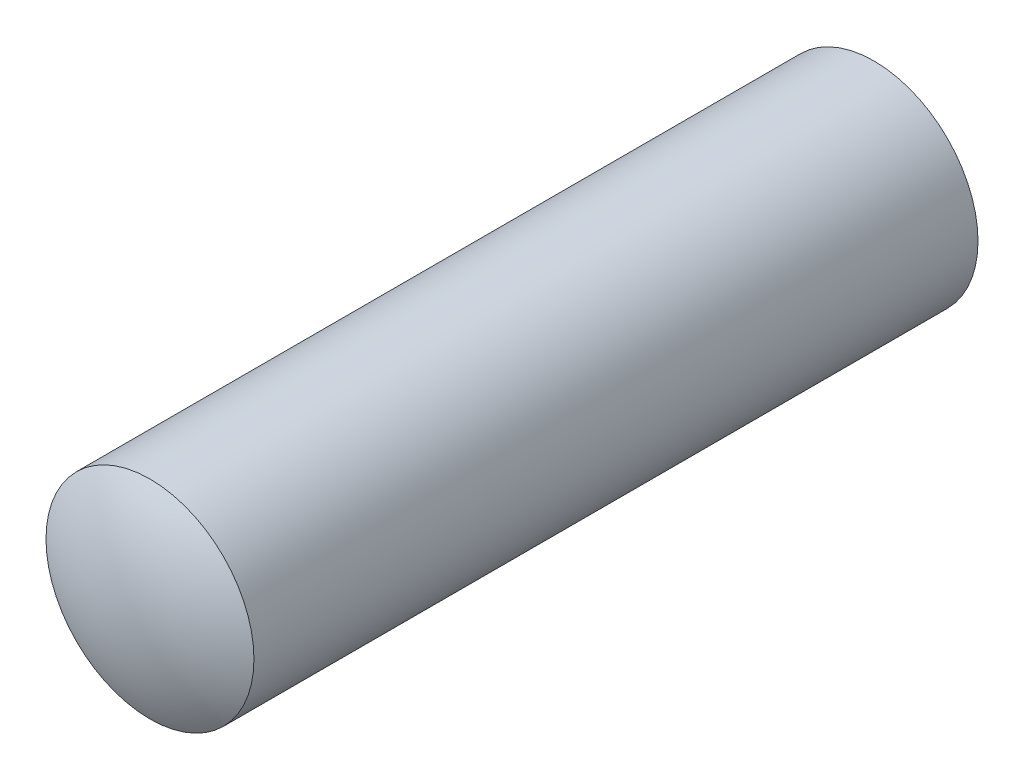
SolidWorks part; units mm, degrees
ref_plane "Front" through (0, 0, 0) normal (0, 0, 1) x (1, 0, 0)
ref_plane "Top" through (0, 0, 0) normal (0, 1, 0) x (1, 0, 0)
ref_plane "Right" through (0, 0, 0) normal (1, 0, 0) x (0, 0, -1)
sketch "Logo3_Revol_Axis" plane through (0, 0, 0) normal (0, 1, 0) x (1, 0, 0)
  line L0 (0, -30.1653) -> (0, 30.1653) construction
sketch "Logo3_bib1" plane through (0, 0, 0) normal (0, -1, 0) x (-1, 0, 0)
  line L0 (0, 8) -> (0, -7)
  line L1 (2, 7.4641) -> (2, -6.4641)
  line L10 (0, 47.5372) -> (0, -34.1764) construction
  arc A0 (2, 7.4641) -> (0, 8) centre (0, 4) ccw
  arc A1 (0, -7) -> (2, -6.4641) centre (0, -3) ccw
revolve "Revolve1" add sketch "Logo3_bib1" angle 360 about L10
equation "\"ray2@XZQB7_bib1\" = \"XZQB7_d1@XZQB7_bib1\""
equation "\"Ray1@XZQB7_bib1\" = \"XZQB7_d1@XZQB7_bib1\""
equation "\"dia1@XZQB7_bib1\" = \"XZQB7_d1@XZQB7_bib1\"/2"
